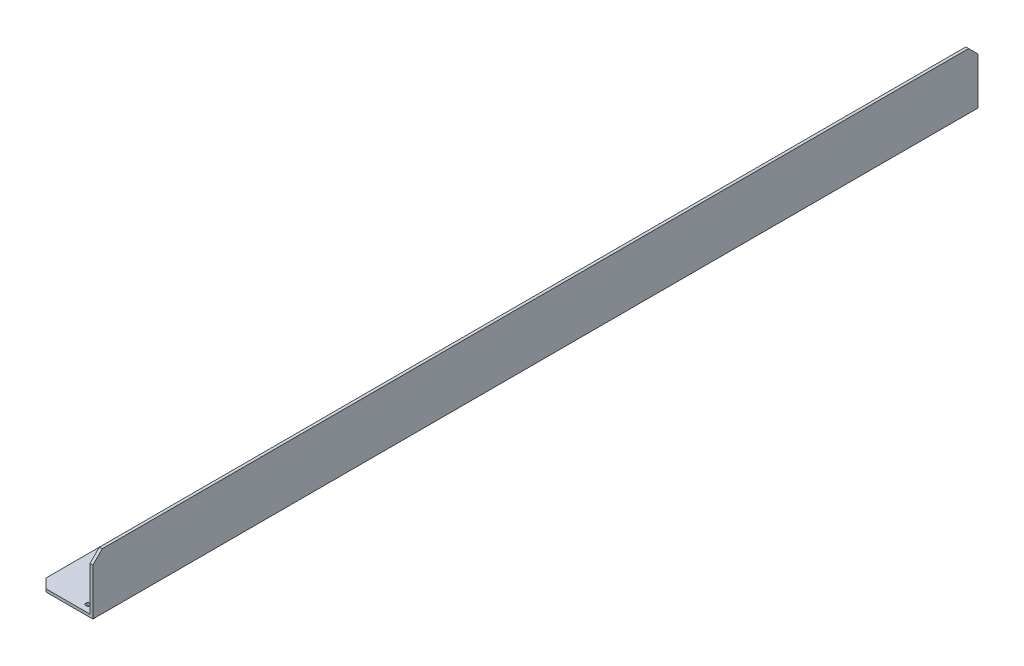
from build123d import *

# Parameters (mm, degrees)
EXTRUDE_1_DEPTH    = 472.5
HOLE_WIZARD_M4_1_D = 4.8
CHAMFER_1_SIZE     = 10
HOLE_WIZARD_M5_1_D = 4.2


with BuildPart() as part:
    # 草图1 → 凸台-拉伸1 (new, symmetric)
    with BuildSketch(Plane.XY):
        Polygon((0, 0), (60, 0), (60, 60), (57, 60), (57, 3), (0, 3), align=None)
    extrude(amount=EXTRUDE_1_DEPTH, both=True)

    # M4 间隙孔1 (through all)
    with Locations(Plane(origin=(0, 3, 0), x_dir=(1, 0, 0), z_dir=(0, 1, 0))):
        with Locations((47, 0), (47, 232.25), (47, 464.5), (47, -464.5), (47, -232.25), (47, 449.5), (47, -449.5)):
            Hole(HOLE_WIZARD_M4_1_D / 2)

    # 倒角1
    chamfer_1_edges = [part.edges().sort_by_distance(p)[0] for p in [
        (58.5, 60, 472.5),
        (0, 1.5, 472.5),
        (58.5, 60, -472.5),
        (0, 1.5, -472.5),
    ]]
    chamfer(chamfer_1_edges, length=CHAMFER_1_SIZE)

    # M5 螺纹孔1 (through all)
    with Locations(Plane(origin=(0, 3, 0), x_dir=(1, 0, 0), z_dir=(0, 1, 0))):
        with Locations((9.75, 373.7), (39.75, 373.7), (24.75, 358.7), (9.75, 358.7), (39.75, 358.7), (24.75, 373.7)):
            Hole(HOLE_WIZARD_M5_1_D / 2)


solid = part.part
